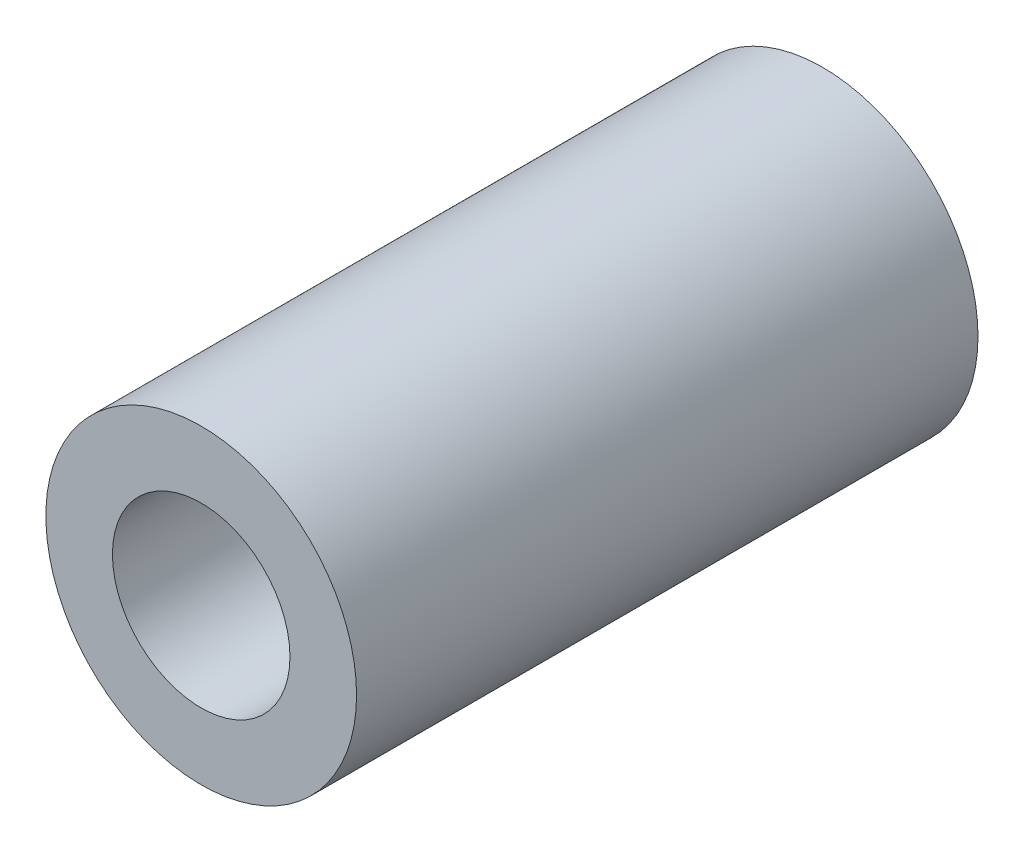
SolidWorks part; units mm, degrees
ref_plane "Front Plane" through (0, 0, 0) normal (0, 0, 1) x (1, 0, 0)
ref_plane "Top Plane" through (0, 0, 0) normal (0, 1, 0) x (1, 0, 0)
ref_plane "Right Plane" through (0, 0, 0) normal (1, 0, 0) x (0, 0, -1)
sketch "Sketch1" plane through (0, 0, 0) normal (0, 0, 1) x (1, 0, 0)
  circle A0 centre (0, 0) radius 7
  circle A1 centre (0, 0) radius 4
  dimension "D1" = 14
  dimension "D2" = 8
extrude "Boss-Extrude1" add sketch "Sketch1" against normal blind 28
